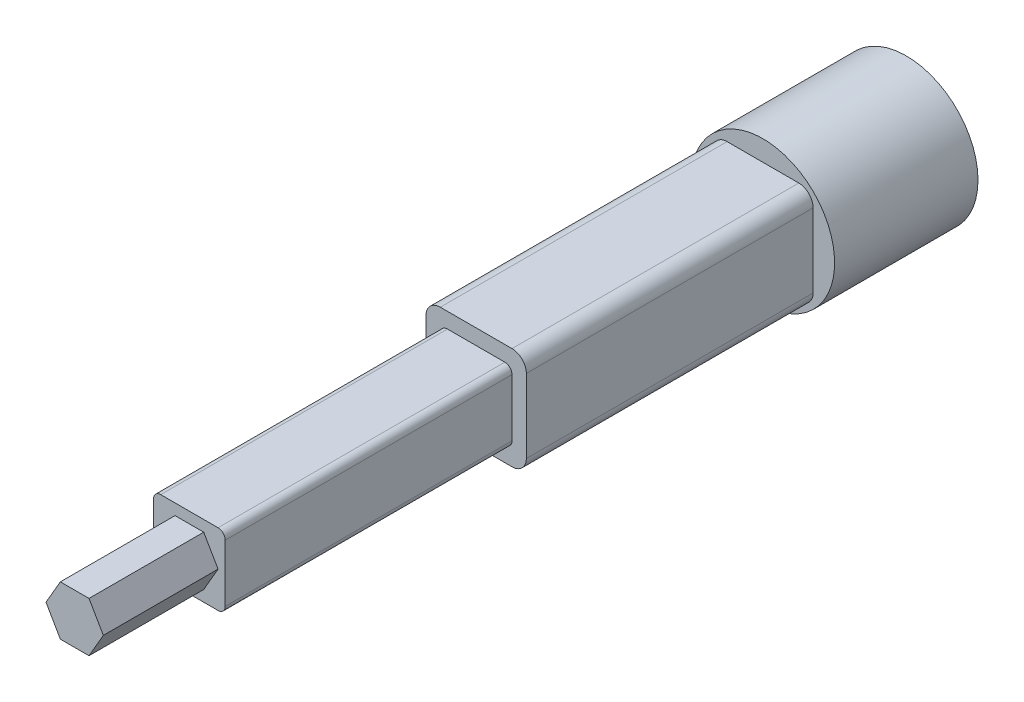
from build123d import *

# Parameters (mm, degrees)
SKETCH1_R           = 5
BOSS_EXTRUDE1_DEPTH = 10
SKETCH2_W           = 7
SKETCH2_H           = 7.141428428
BOSS_EXTRUDE2_DEPTH = 20
FILLET1_R           = 1
SKETCH3_W           = 5
SKETCH3_H           = 5
BOSS_EXTRUDE3_DEPTH = 20
FILLET2_R           = 0.5
BOSS_EXTRUDE4_DEPTH = 8


with BuildPart() as part:
    # Sketch1 → Boss-Extrude1 (new body)
    with BuildSketch(Plane.XY):
        Circle(SKETCH1_R)
    extrude(amount=BOSS_EXTRUDE1_DEPTH)

    # Sketch2 → Boss-Extrude2 (add)
    with BuildSketch(Plane.XY.offset(10)):
        Rectangle(SKETCH2_W, SKETCH2_H)
    extrude(amount=BOSS_EXTRUDE2_DEPTH)

    # Fillet1
    fillet1_edges = [part.edges().sort_by_distance(p)[0] for p in [
        (3.5, -3.570714214, 20),
        (3.5, 3.570714214, 20),
        (-3.5, 3.570714214, 20),
        (-3.5, -3.570714214, 20),
    ]]
    fillet(fillet1_edges, radius=FILLET1_R)

    # Sketch3 → Boss-Extrude3 (add)
    with BuildSketch(Plane.XY.offset(30)):
        Rectangle(SKETCH3_W, SKETCH3_H)
    extrude(amount=BOSS_EXTRUDE3_DEPTH)

    # Fillet2
    fillet2_edges = [part.edges().sort_by_distance(p)[0] for p in [
        (-2.5, 2.5, 40),
        (-2.5, -2.5, 40),
        (2.5, -2.5, 40),
        (2.5, 2.5, 40),
    ]]
    fillet(fillet2_edges, radius=FILLET2_R)

    # Sketch4 → Boss-Extrude4 (add)
    with BuildSketch(Plane.XY.offset(50)):
        Polygon((1, 1.732050808), (-1, 1.732050808), (-2, 0), (-1, -1.732050808), (1, -1.732050808), (2, 0), align=None)
    extrude(amount=BOSS_EXTRUDE4_DEPTH)


solid = part.part
